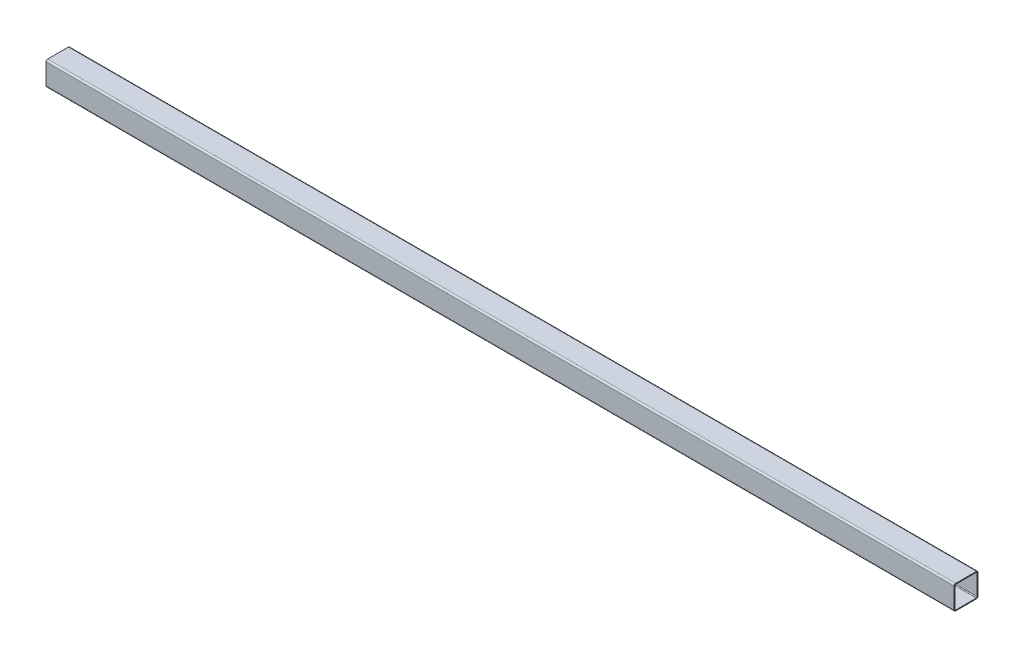
from build123d import *

# Parameters (mm, degrees)
GB_6728_1986_150_X_150_X_5_1_DEPTH = 5700


with BuildPart() as part:
    # Sketch1 → Gb／6728-1986方形空心型钢 150 X 150 X 5(1) (new body)
    with BuildSketch(Plane.YZ.offset(-2850)):
        with BuildLine():
            Line((-65, -75), (65, -75))
            ThreePointArc((65, -75), (72.071067812, -72.071067812), (75, -65))
            Line((75, -65), (75, 65))
            ThreePointArc((75, 65), (72.071067812, 72.071067812), (65, 75))
            Line((65, 75), (-65, 75))
            ThreePointArc((-65, 75), (-72.071067812, 72.071067812), (-75, 65))
            Line((-75, 65), (-75, -65))
            ThreePointArc((-75, -65), (-72.071067812, -72.071067812), (-65, -75))
        make_face()
        with BuildLine():
            Line((-65, -70), (65, -70))
            ThreePointArc((65, -70), (68.535533906, -68.535533906), (70, -65))
            Line((70, -65), (70, 65))
            ThreePointArc((70, 65), (68.535533906, 68.535533906), (65, 70))
            Line((65, 70), (-65, 70))
            ThreePointArc((-65, 70), (-68.535533906, 68.535533906), (-70, 65))
            Line((-70, 65), (-70, -65))
            ThreePointArc((-70, -65), (-68.535533906, -68.535533906), (-65, -70))
        make_face(mode=Mode.SUBTRACT)
    extrude(amount=GB_6728_1986_150_X_150_X_5_1_DEPTH)


solid = part.part
